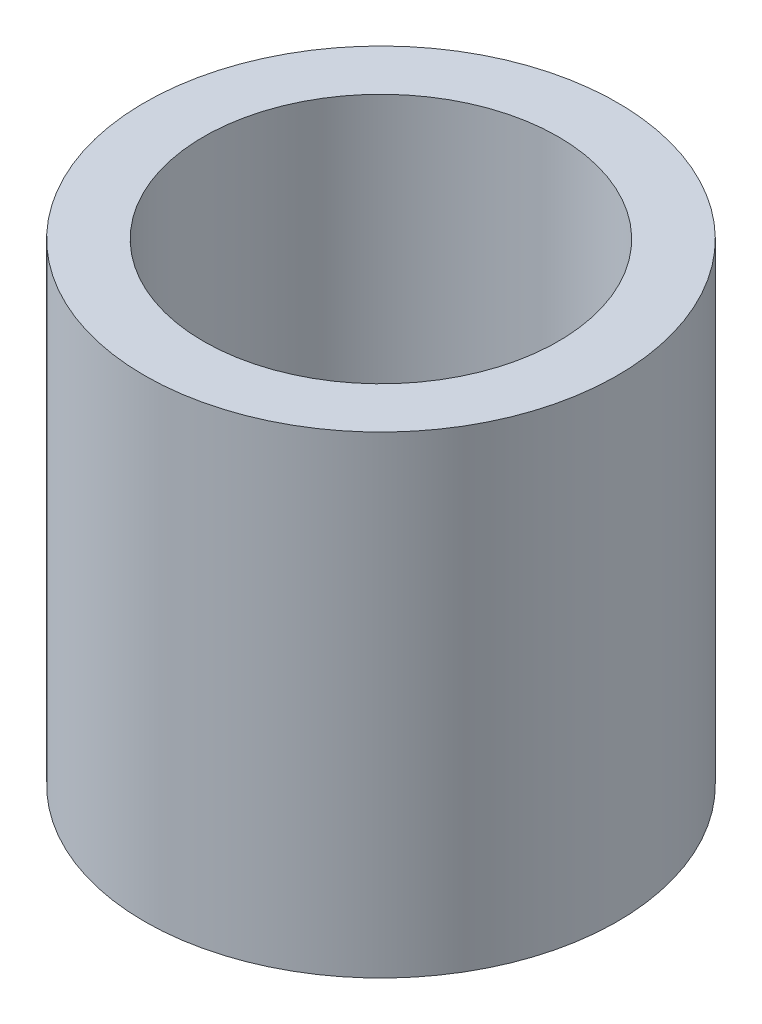
SolidWorks part; units mm, degrees
ref_plane "前视基准面" through (0, 0, 0) normal (0, 0, 1) x (1, 0, 0)
ref_plane "上视基准面" through (0, 0, 0) normal (0, 1, 0) x (1, 0, 0)
ref_plane "右视基准面" through (0, 0, 0) normal (1, 0, 0) x (0, 0, -1)
sketch "草图1" plane through (0, 0, 0) normal (0, 1, 0) x (1, 0, 0)
  circle A0 centre (0, 0) radius 7.5
  circle A1 centre (0, 0) radius 10
  dimension "D1" = 15
  dimension "D2" = 20
extrude "凸台-拉伸1" add sketch "草图1" along normal mid plane 20
